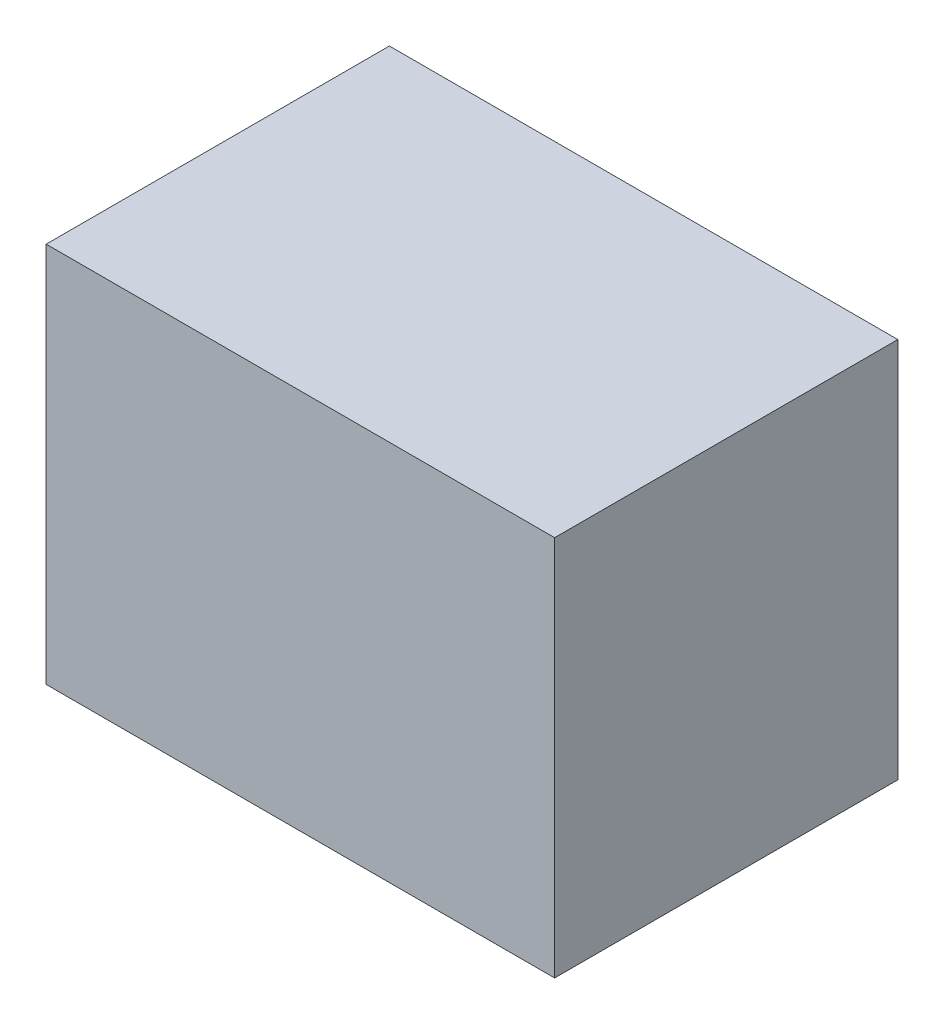
from build123d import *

# Parameters (mm, degrees)
SKETCH1_W           = 40
SKETCH1_H           = 30
BOSS_EXTRUDE1_DEPTH = 27


with BuildPart() as part:
    # Sketch1 → Boss-Extrude1 (new body)
    with BuildSketch(Plane.XY):
        Rectangle(SKETCH1_W, SKETCH1_H)
    extrude(amount=BOSS_EXTRUDE1_DEPTH)


solid = part.part
